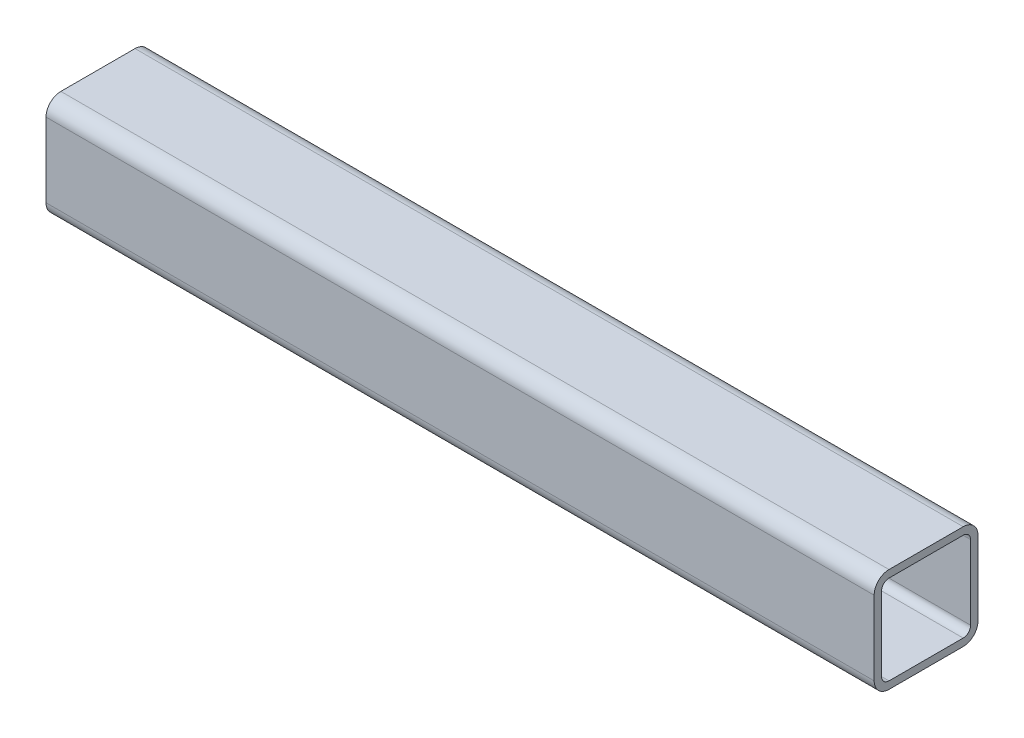
from build123d import *

# Parameters (mm, degrees)
BOSS_EXTRUDE1_DEPTH = 638


with BuildPart() as part:
    # Sketch1 → Boss-Extrude1 (new body)
    with BuildSketch(Plane(origin=(249, 0, 0), x_dir=(0, 0, -1), z_dir=(1, 0, 0))):
        with BuildLine():
            Line((40, -28.571428571), (40, 28.571428571))
            ThreePointArc((40, 28.571428571), (36.652648928, 36.652648928), (28.571428571, 40))
            Line((28.571428571, 40), (-28.571428571, 40))
            ThreePointArc((-28.571428571, 40), (-36.652648928, 36.652648928), (-40, 28.571428571))
            Line((-40, 28.571428571), (-40, -28.571428571))
            ThreePointArc((-40, -28.571428571), (-36.652648928, -36.652648928), (-28.571428571, -40))
            Line((-28.571428571, -40), (28.571428571, -40))
            ThreePointArc((28.571428571, -40), (36.652648928, -36.652648928), (40, -28.571428571))
        make_face()
        with BuildLine():
            Line((-34.285714286, -28.571428571), (-34.285714286, 28.571428571))
            ThreePointArc((-34.285714286, 28.571428571), (-32.61203875, 32.61203875), (-28.571428571, 34.285714286))
            Line((-28.571428571, 34.285714286), (28.571428571, 34.285714286))
            ThreePointArc((28.571428571, 34.285714286), (32.61203875, 32.61203875), (34.285714286, 28.571428571))
            Line((34.285714286, 28.571428571), (34.285714286, -28.571428571))
            ThreePointArc((34.285714286, -28.571428571), (32.61203875, -32.61203875), (28.571428571, -34.285714286))
            Line((28.571428571, -34.285714286), (-28.571428571, -34.285714286))
            ThreePointArc((-28.571428571, -34.285714286), (-32.61203875, -32.61203875), (-34.285714286, -28.571428571))
        make_face(mode=Mode.SUBTRACT)
    extrude(amount=-BOSS_EXTRUDE1_DEPTH)


solid = part.part
